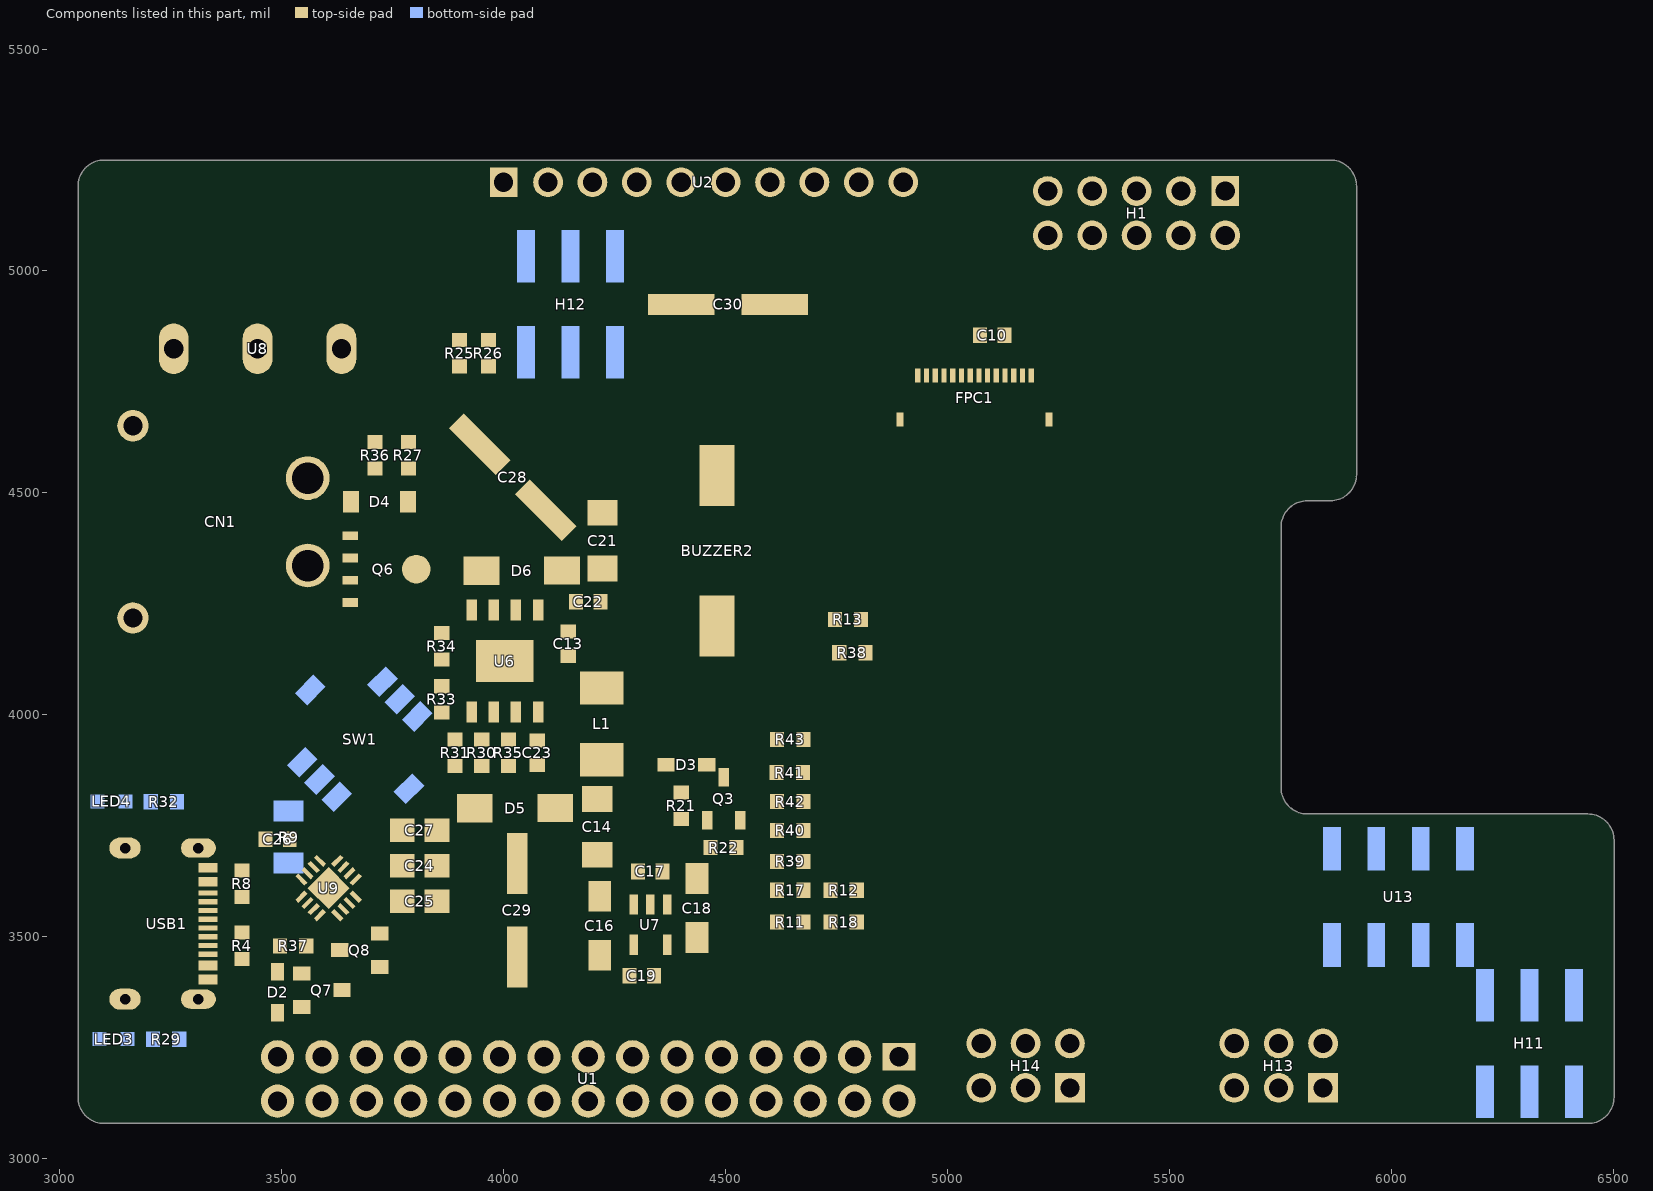
[diagram p0: the components of this part, seen from the top]
# Altium PCB MISC51977.pcbdoc (part 4 of 4)
Units mil, origin at the board's own origin, x right, y up, seen from the top; angles counter-clockwise.
Board outline 3460 x 2170.19 mil, 4 copper layers (Top Layer, VCC, GND, Bottom Layer), stack 62.447 mil thick; 74 components, 60 nets, 282 pads, 462 vias.

## Other copper (continued)
Bottom Layer:
  region net $2N1757: 3177.91,3809.54 3177.91,3799.54 3174.46,3799.22 3171.12,3798.27 3168.01,3796.71 3165.25,3794.61 3162.91,3792.04 3162.91,3817.04 3165.25,3814.47 3168.01,3812.37 3171.12,3810.82 3174.46,3809.86 3177.91,3809.54
  region net $1N29256: 3182.91,3274.92 3182.91,3264.92 3179.46,3264.6 3176.12,3263.64 3173.01,3262.09 3170.25,3259.99 3167.91,3257.42 3167.91,3282.42 3170.25,3279.84 3173.01,3277.74 3176.12,3276.19 3179.46,3275.24 3182.91,3274.92
  region net +5V: 3299.6,3275 3299.6,3265 3296.15,3264.68 3292.81,3263.72 3289.7,3262.17 3286.94,3260.07 3284.6,3257.5 3284.6,3282.5 3286.94,3279.93 3289.7,3277.83 3292.81,3276.28 3296.15,3275.32 3299.6,3275
  region net $1N29256: 3178.53,3264.92 3178.53,3274.92 3181.99,3275.24 3185.33,3276.19 3188.44,3277.74 3191.2,3279.84 3193.53,3282.42 3193.53,3257.42 3191.2,3259.99 3188.44,3262.09 3185.33,3263.64 3181.99,3264.6 3178.53,3264.92
  region net $2N1757: 3173.53,3799.54 3173.53,3809.54 3176.99,3809.86 3180.33,3810.82 3183.44,3812.37 3186.2,3814.47 3188.53,3817.04 3188.53,3792.04 3186.2,3794.61 3183.44,3796.71 3180.33,3798.27 3176.99,3799.22 3173.53,3799.54
  region net 3V3: 3278.97,3826.85 3284.91,3818.65 3282.63,3815.05 3280.97,3811.12 3279.95,3806.99 3279.6,3802.74 3263.06,3821.55 3267.31,3821.89 3271.44,3822.91 3275.37,3824.58 3278.97,3826.85
  region net TX: 4750.32,3262.61 4757.39,3269.68 4759.59,3267.66 4761.66,3266.14 4763.63,3265.04 4765.52,3264.33 4767.36,3263.95 4769.18,3263.86 4771.01,3264 4772.86,3264.32 4776.78,3265.3 4781.14,3266.41 4783.56,3266.87 4786.17,3267.22 4789,3267.39 4792.08,3267.34 4752.66,3227.92 4752.61,3231 4752.78,3233.83 4753.13,3236.44 4753.59,3238.86 4754.7,3243.22 4755.68,3247.14 4756,3248.99 4756.14,3250.82 4756.05,3252.64 4755.67,3254.48 4754.96,3256.37 4753.86,3258.34 4752.34,3260.41
  region net RX: 4732.05,3215.02 4738.75,3194.18 4736.84,3195.89 4734.85,3197.27 4732.8,3198.34 4730.69,3199.13 4728.53,3199.66 4726.31,3199.95 4724.05,3200.03 4721.74,3199.91 4717.01,3199.17 4712.16,3197.93 4707.21,3196.36 4702.19,3194.64 4723.78,3246.05 4724.63,3244.01 4725.27,3241.95 4726.05,3237.82 4726.42,3233.7 4726.67,3229.65 4727.06,3225.71 4727.41,3223.79 4727.9,3221.93 4728.58,3220.11 4729.47,3218.35 4730.61,3216.65
  region net MOTOR_DIR_L: 4550.32,3162.61 4557.39,3169.68 4559.59,3167.66 4561.66,3166.14 4563.63,3165.04 4565.52,3164.33 4567.36,3163.95 4569.18,3163.86 4571.01,3164 4572.86,3164.32 4576.78,3165.3 4581.14,3166.41 4583.56,3166.87 4586.17,3167.22 4589,3167.39 4592.08,3167.34 4552.66,3127.92 4552.61,3131 4552.78,3133.83 4553.13,3136.44 4553.59,3138.86 4554.7,3143.22 4555.68,3147.14 4556,3148.99 4556.14,3150.82 4556.05,3152.64 4555.67,3154.48 4554.96,3156.37 4553.86,3158.34 4552.34,3160.41
  region net MOTOR_DIR_R: 4450.32,3162.61 4457.39,3169.68 4459.59,3167.66 4461.66,3166.14 4463.63,3165.04 4465.52,3164.33 4467.36,3163.95 4469.18,3163.86 4471.01,3164 4472.86,3164.32 4476.78,3165.3 4481.14,3166.41 4483.56,3166.87 4486.17,3167.22 4489,3167.39 4492.08,3167.34 4452.66,3127.92 4452.61,3131 4452.78,3133.83 4453.13,3136.44 4453.59,3138.86 4454.7,3143.22 4455.68,3147.14 4456,3148.99 4456.14,3150.82 4456.05,3152.64 4455.67,3154.48 4454.96,3156.37 4453.86,3158.34 4452.34,3160.41
  region net TFT180_DC: 4350.32,3162.61 4357.39,3169.68 4359.59,3167.66 4361.66,3166.14 4363.63,3165.04 4365.52,3164.33 4367.36,3163.95 4369.18,3163.86 4371.01,3164 4372.86,3164.32 4376.78,3165.3 4381.14,3166.41 4383.56,3166.87 4386.17,3167.22 4389,3167.39 4392.08,3167.34 4352.66,3127.92 4352.61,3131 4352.78,3133.83 4353.13,3136.44 4353.59,3138.86 4354.7,3143.22 4355.68,3147.14 4356,3148.99 4356.14,3150.82 4356.05,3152.64 4355.67,3154.48 4354.96,3156.37 4353.86,3158.34 4352.34,3160.41
  region net TFT180_RES: 4250.32,3262.61 4257.39,3269.68 4259.59,3267.66 4261.66,3266.14 4263.63,3265.04 4265.52,3264.33 4267.36,3263.95 4269.18,3263.86 4271.01,3264 4272.86,3264.32 4276.78,3265.3 4281.14,3266.41 4283.56,3266.87 4286.17,3267.22 4289,3267.39 4292.08,3267.34 4252.66,3227.92 4252.61,3231 4252.78,3233.83 4253.13,3236.44 4253.59,3238.86 4254.7,3243.22 4255.68,3247.14 4256,3248.99 4256.14,3250.82 4256.05,3252.64 4255.67,3254.48 4254.96,3256.37 4253.86,3258.34 4252.34,3260.41
  region net TFT180_SCL: 3850.32,3262.61 3857.39,3269.68 3859.59,3267.66 3861.66,3266.14 3863.63,3265.04 3865.52,3264.33 3867.36,3263.95 3869.18,3263.86 3871.01,3264 3872.86,3264.32 3876.78,3265.3 3881.14,3266.41 3883.56,3266.87 3886.17,3267.22 3889,3267.39 3892.08,3267.34 3852.66,3227.92 3852.61,3231 3852.78,3233.83 3853.13,3236.44 3853.59,3238.86 3854.7,3243.22 3855.68,3247.14 3856,3248.99 3856.14,3250.82 3856.05,3252.64 3855.67,3254.48 3854.96,3256.37 3853.86,3258.34 3852.34,3260.41
  region net TFT180_CS: 3750.32,3262.61 3757.39,3269.68 3759.59,3267.66 3761.66,3266.14 3763.63,3265.04 3765.52,3264.33 3767.36,3263.95 3769.18,3263.86 3771.01,3264 3772.86,3264.32 3776.78,3265.3 3781.14,3266.41 3783.56,3266.87 3786.17,3267.22 3789,3267.39 3792.08,3267.34 3752.66,3227.92 3752.61,3231 3752.78,3233.83 3753.13,3236.44 3753.59,3238.86 3754.7,3243.22 3755.68,3247.14 3756,3248.99 3756.14,3250.82 3756.05,3252.64 3755.67,3254.48 3754.96,3256.37 3753.86,3258.34 3752.34,3260.41
  region net MOTOR_PWM_R: 3622.61,3169.68 3629.68,3162.61 3627.66,3160.41 3626.14,3158.34 3625.04,3156.37 3624.33,3154.48 3623.95,3152.64 3623.86,3150.82 3624,3148.99 3624.32,3147.14 3625.3,3143.22 3626.41,3138.86 3626.87,3136.44 3627.22,3133.83 3627.39,3131 3627.34,3127.92 3587.92,3167.34 3591,3167.39 3593.83,3167.22 3596.44,3166.87 3598.86,3166.41 3603.22,3165.3 3607.14,3164.32 3608.99,3164 3610.82,3163.86 3612.64,3163.95 3614.48,3164.33 3616.37,3165.04 3618.34,3166.14 3620.41,3167.66
  region net TX: 5829.92,3693.27 5829.92,3703.27 5833.38,3703.6 5836.72,3704.55 5839.82,3706.1 5842.59,3708.2 5844.92,3710.77 5844.92,3685.77 5842.59,3688.35 5839.82,3690.45 5836.72,3692 5833.38,3692.95 5829.92,3693.27
  region net RX: 5933.62,3639.15 5937.03,3656.7 5939.61,3659.64 5941.81,3662.87 5943.59,3666.35 5944.92,3670.03 5944.92,3649.06 5939.11,3644.29 5933.62,3639.15
  region net ENCODER_PWM_R: 5139.13,3288.8 5146.2,3295.87 5148.12,3294.11 5149.94,3292.77 5151.67,3291.79 5153.35,3291.15 5154.99,3290.78 5156.61,3290.67 5158.24,3290.75 5159.89,3290.99 5163.39,3291.77 5167.26,3292.66 5171.69,3293.32 5174.17,3293.46 5176.86,3293.41 5141.59,3258.14 5141.54,3260.83 5141.68,3263.31 5142.34,3267.74 5143.23,3271.61 5144.01,3275.11 5144.25,3276.76 5144.33,3278.39 5144.22,3280.01 5143.85,3281.65 5143.21,3283.33 5142.23,3285.06 5140.89,3286.88
  region net $1N14385: 6384.62,3203.31 6385.98,3216.09 6389.59,3213.81 6393.51,3212.15 6397.65,3211.13 6401.89,3210.78 6389.92,3187.4 6389.58,3191.65 6388.56,3195.79 6386.89,3199.71 6384.62,3203.31
  region net $1N4273: 6376.73,3358.27 6376.73,3368.27 6379.88,3368.6 6382.9,3369.56 6385.65,3371.13 6388.03,3373.23 6389.92,3375.77 6389.92,3350.77 6388.03,3353.31 6385.65,3355.41 6382.9,3356.98 6379.88,3357.94 6376.73,3358.27
  region net $1N14409: 6184.62,3203.31 6185.98,3216.09 6189.59,3213.81 6193.51,3212.15 6197.65,3211.13 6201.89,3210.78 6189.92,3187.4 6189.58,3191.65 6188.56,3195.79 6186.89,3199.71 6184.62,3203.31
  region net $1N14395: 6174.92,3358.27 6174.92,3368.27 6178.38,3368.59 6181.72,3369.55 6184.82,3371.1 6187.59,3373.2 6189.92,3375.77 6189.92,3350.77 6187.59,3353.34 6184.82,3355.44 6181.72,3356.99 6178.38,3357.95 6174.92,3358.27
  region net $1N45238: 4014.92,4839.37 4014.92,4849.37 4018.38,4849.69 4021.72,4850.64 4024.82,4852.19 4027.59,4854.29 4029.92,4856.87 4029.92,4831.87 4027.59,4834.44 4024.82,4836.54 4021.72,4838.09 4018.38,4839.04 4014.92,4839.37
  region net $1N45237: 4030.98,4968.91 4024.62,4976.69 4026.89,4980.29 4028.56,4984.21 4029.58,4988.35 4029.92,4992.6 4046.89,4974.22 4042.65,4973.87 4038.51,4972.85 4034.59,4971.19 4030.98,4968.91
  region net KEY_UP: 3724.7,4037.31 3714.7,4037 3713.76,4041.16 3712.16,4045.11 3709.96,4048.76 3707.2,4052 3732.2,4052.31 3729.44,4049.06 3727.23,4045.41 3725.64,4041.46 3724.7,4037.31
  region net KEY_UP: 3760.76,4089.45 3766.84,4079.45 3762.69,4078.51 3758.73,4076.92 3755.09,4074.71 3751.84,4071.95 3745.76,4096.95 3749.01,4094.19 3752.65,4091.99 3756.61,4090.39 3760.76,4089.45
  region net KEY_LEFT: 3845.21,4005 3838.29,3995 3834.14,3994.06 3830.18,3992.47 3826.54,3990.26 3823.29,3987.5 3830.21,4012.5 3833.46,4009.74 3837.11,4007.53 3841.06,4005.94 3845.21,4005
  region net KEY_DOWN: 3664.54,3807.53 3657.47,3800.46 3654.8,3802.68 3651.76,3804.37 3648.47,3805.46 3645.03,3805.94 3641.56,3805.76 3658.3,3822.51 3658.58,3819.2 3659.36,3815.97 3660.64,3812.89 3662.38,3810.06 3664.54,3807.53
  region net KEY_MID: 3618.79,3869.53 3624.87,3859.53 3620.72,3858.59 3616.76,3857 3613.12,3854.79 3609.87,3852.03 3603.79,3877.03 3607.03,3874.27 3610.68,3872.06 3614.63,3870.47 3618.79,3869.53
  region net KEY_RIGHT: 3579.81,3908.5 3585.89,3898.5 3581.73,3897.56 3577.78,3895.96 3574.13,3893.76 3570.89,3891 3564.81,3916 3568.05,3913.24 3571.7,3911.03 3575.65,3909.44 3579.81,3908.5
  region net UD+: 3285,3521.33 3275,3521.33 3274.82,3523.1 3274.31,3525.04 3273.53,3526.87 3272.55,3528.33 3287.45,3528.33 3286.47,3526.87 3285.69,3525.04 3285.18,3523.1
  region net TX: 3605.61,3701.2 3612.68,3694.13 3611.56,3692.75 3610.55,3691.02 3609.81,3689.18 3609.46,3687.45 3598.92,3697.99 3600.65,3698.33 3602.5,3699.08 3604.23,3700.08
  region net $1N5665: 3663.19,3396.41 3678.19,3396.41 3678.1,3394.02 3678.07,3391.88 3678.19,3390.88 3678.46,3389.91 3678.93,3388.95 3679.64,3388.01 3661.74,3388.01 3662.45,3388.95 3662.92,3389.91 3663.19,3390.88 3663.31,3391.88 3663.28,3394.02
  region net $1N5665: 3678.19,3431.99 3663.19,3425.65 3663.28,3427.09 3663.49,3428.44 3663.86,3430.84 3663.84,3431.86 3663.54,3432.75 3662.87,3433.48 3661.74,3434.05 3677.19,3441.92 3676.95,3440.72 3676.94,3439.5 3677.33,3437.01 3677.9,3434.49
  region net KEY_DOWN: 4256.83,3373.49 4246.83,3373.49 4246.65,3375.26 4246.14,3377.19 4245.36,3379.03 4244.38,3380.49 4259.29,3380.49 4258.3,3379.03 4257.53,3377.19 4257.02,3375.26
  region net KEY_DOWN: 4260,3513.67 4270,3513.67 4270.18,3511.9 4270.69,3509.96 4271.47,3508.13 4272.45,3506.67 4257.55,3506.67 4258.53,3508.13 4259.31,3509.96 4259.82,3511.9
  region net MOTOR_PWM_R: 4003.06,3304.36 3995.99,3311.43 3997.11,3312.81 3998.12,3314.54 3998.86,3316.38 3999.2,3318.11 4009.75,3307.57 4008.02,3307.23 4006.17,3306.49 4004.44,3305.48
  region net MOTOR_PWM_R: 4556.33,3595 4556.33,3605 4558.1,3605.18 4560.04,3605.69 4561.87,3606.47 4563.33,3607.45 4563.33,3592.55 4561.87,3593.53 4560.04,3594.31 4558.1,3594.82
  region net KEY_DOWN: 4516.93,3851.8 4509.86,3858.87 4510.98,3860.25 4511.99,3861.98 4512.73,3863.83 4513.08,3865.56 4523.62,3855.02 4521.89,3854.67 4520.04,3853.93 4518.31,3852.92
  region net KEY_UP: 3714.7,4008.44 3724.7,4008.89 3724.89,4007.11 3725.41,4005.17 3726.22,4003.34 3727.25,4001.89 3712.35,4001.44 3713.29,4002.91 3714.03,4004.75 3714.52,4006.68
  region net KEY_RIGHT: 4631.81,3899.09 4638.88,3906.16 4640.26,3905.04 4641.99,3904.03 4643.84,3903.29 4645.57,3902.94 4635.03,3892.4 4634.68,3894.13 4633.94,3895.98 4632.93,3897.71
  region net KEY_MID: 4563.17,3849.76 4570.19,3856.88 4571.57,3855.76 4573.3,3854.75 4575.15,3854.01 4576.89,3853.68 4566.4,3843.09 4566.05,3844.81 4565.3,3846.65 4564.29,3848.38
  region net $1N45238: 4019.73,4849.37 4019.73,4839.37 4017.96,4839.18 4016.02,4838.67 4014.19,4837.89 4012.73,4836.91 4012.73,4851.82 4014.19,4850.84 4016.02,4850.06 4017.96,4849.55
  region net $1N45237: 3956.13,4908.2 3963.2,4901.13 3962.08,4899.75 3961.07,4898.02 3960.33,4896.17 3959.98,4894.44 3949.44,4904.98 3951.17,4905.33 3953.02,4906.07 3954.75,4907.08
  region net I2C_SCL: 5546.33,4760 5546.33,4770 5548.1,4770.18 5550.04,4770.69 5551.87,4771.47 5553.33,4772.45 5553.33,4757.55 5551.87,4758.53 5550.04,4759.31 5548.1,4759.82
  region net $1N14385: 4689.97,3504.64 4689.97,3494.64 4688.2,3494.46 4686.26,3493.95 4684.43,3493.17 4682.97,3492.19 4682.97,3507.09 4684.43,3506.11 4686.26,3505.33 4688.2,3504.82
  region net $1N4273: 6389.86,3368.27 6387.28,3358.27 6385.55,3358.15 6383.66,3357.8 6381.82,3357.24 6380.28,3356.51 6382.86,3371.19 6383.48,3370.53 6384.23,3369.95 6386.02,3369.04 6387.97,3368.47
  region net $1N14395: 6169.65,3368.27 6169.65,3358.27 6167.88,3358.09 6165.95,3357.58 6164.11,3356.8 6162.65,3355.82 6162.65,3370.72 6164.11,3369.74 6165.95,3368.96 6167.88,3368.45
  region net $1N14385: 6268.67,3230 6268.67,3220 6266.9,3219.82 6264.96,3219.31 6263.13,3218.53 6261.67,3217.55 6261.67,3232.45 6263.13,3231.47 6264.96,3230.69 6266.9,3230.18
  region net $1N14385: 4881.61,3494.64 4881.07,3504.64 4882.86,3504.83 4884.8,3505.36 4886.62,3506.17 4888.07,3507.21 4888.61,3492.31 4887.13,3493.24 4885.29,3493.98 4883.36,3494.47
  region net +5V: 3296.33,3265 3296.33,3275 3298.1,3275.18 3300.04,3275.69 3301.87,3276.47 3303.33,3277.45 3303.33,3262.55 3301.87,3263.53 3300.04,3264.31 3298.1,3264.82
  region net KEY_UP: 4736.33,3950 4736.33,3960 4738.1,3960.18 4740.04,3960.69 4741.87,3961.47 4743.33,3962.45 4743.33,3947.55 4741.87,3948.53 4740.04,3949.31 4738.1,3949.82
  region net I2C_SDA: 4695,4003.67 4705,4003.67 4705.18,4001.9 4705.69,3999.96 4706.47,3998.13 4707.45,3996.67 4692.55,3996.67 4693.53,3998.13 4694.31,3999.96 4694.82,4001.9
  region net GND: 4033.67,3400 4033.67,3390 4031.9,3389.82 4029.96,3389.31 4028.13,3388.53 4026.67,3387.55 4026.67,3402.45 4028.13,3401.47 4029.96,3400.69 4031.9,3400.18
  region net 3V3: 3297.71,3831.45 3291.25,3839.13 3292.36,3840.48 3293.39,3842.18 3294.19,3843.98 3294.61,3845.67 3304.52,3834.54 3302.75,3834.28 3300.88,3833.58 3299.12,3832.59
  region net AGND: 3478.67,3535 3478.67,3525 3476.9,3524.82 3474.96,3524.31 3473.13,3523.53 3471.67,3522.55 3471.67,3537.45 3473.13,3536.47 3474.96,3535.69 3476.9,3535.18
  region net GND: 3508.67,3485 3508.67,3475 3506.9,3474.82 3504.96,3474.31 3503.13,3473.53 3501.67,3472.55 3501.67,3487.45 3503.13,3486.47 3504.96,3485.69 3506.9,3485.18
  region net AGND: 3727.15,3621.33 3717.15,3621.33 3716.96,3623.1 3716.45,3625.04 3715.68,3626.87 3714.69,3628.33 3729.6,3628.33 3728.62,3626.87 3727.84,3625.04 3727.33,3623.1
  region net AGND: 3727.15,3584.39 3717.15,3584.39 3716.96,3586.16 3716.45,3588.1 3715.68,3589.93 3714.69,3591.39 3729.6,3591.39 3728.62,3589.93 3727.84,3588.1 3727.33,3586.16
  region net AGND: 3717.15,3611.73 3727.15,3611.73 3727.33,3609.96 3727.84,3608.02 3728.62,3606.19 3729.6,3604.73 3714.69,3604.73 3715.68,3606.19 3716.45,3608.02 3716.96,3609.96
  region net AGND: 3707.32,3555 3707.32,3565 3709.09,3565.18 3711.02,3565.69 3712.85,3566.47 3714.32,3567.45 3714.32,3552.55 3712.85,3553.53 3711.02,3554.31 3709.09,3554.82
  region net AGND: 3717.15,3574.49 3727.15,3572.75 3727.3,3571.03 3727.71,3569.11 3728.35,3567.27 3729.16,3565.75 3714.36,3567.49 3715.51,3568.9 3716.39,3570.7 3716.95,3572.65
  region net GND: 3792.39,3475 3797.68,3485 3801.85,3484.84 3803.72,3484.94 3805.91,3485.42 3799.39,3472.54 3798.92,3473.47 3798.29,3474.14 3797.53,3474.59 3796.65,3474.85 3794.63,3475.02
  region net UD+: 3277.74,3500.19 3288.54,3503.53 3291.1,3501.06 3292.48,3500.01 3294.05,3499.14 3280.46,3493.01 3280.66,3493.97 3280.65,3494.94 3280.46,3495.9 3280.12,3496.85 3279.08,3498.63
  region net TFT180_DC: 5028.87,4686.8 5021.8,4693.87 5022.92,4695.25 5023.93,4696.98 5024.67,4698.83 5025.02,4700.56 5035.56,4690.02 5033.83,4689.67 5031.98,4688.93 5030.25,4687.92
  region net TFT180_CS: 5131.33,4725 5131.33,4735 5133.1,4735.18 5135.04,4735.69 5136.87,4736.47 5138.33,4737.45 5138.33,4722.55 5136.87,4723.53 5135.04,4724.31 5133.1,4724.82
  region net TFFT180_SDA: 5036.33,4805 5036.33,4815 5038.1,4815.18 5040.04,4815.69 5041.87,4816.47 5043.33,4817.45 5043.33,4802.55 5041.87,4803.53 5040.04,4804.31 5038.1,4804.82
  region net I2C_SCL: 4827.71,4200.64 4824.02,4211.09 4825.4,4212.78 4826.51,4214.71 4827.41,4216.77 4828.15,4218.84 4836.98,4203.27 4835.88,4203.41 4834.66,4203.38 4832.06,4202.92 4829.61,4201.97 4828.57,4201.35
  region net I2C_SCL: 4852.49,4224.02 4858.47,4214.02 4857.34,4213.91 4856.13,4213.63 4853.71,4212.58 4851.56,4211.06 4850.71,4210.18 4850.07,4209.24 4844.08,4226.11 4846.09,4225.34 4848.21,4224.67 4850.37,4224.2
  region net I2C_SDA: 4728.07,4155.14 4735.14,4148.07 4734.41,4147.21 4733.79,4146.24 4732.84,4144.02 4732.26,4141.65 4731.99,4139.33 4719.33,4151.99 4721.65,4152.26 4724.02,4152.84 4726.24,4153.79 4727.21,4154.41
  region net KEY_DOWN: 4238.79,3689.14 4243.56,3683.88 4247.79,3678.17 4251.45,3672.07 4254.49,3665.65 4256.88,3658.95 4258.61,3652.06 4259.65,3645.03 4260,3637.93 4270,3635 4270.37,3639.69 4271.47,3644.27 4273.27,3648.62 4275.73,3652.63 4278.79,3656.21 4282.37,3659.27 4286.38,3661.73 4290.73,3663.53 4295.31,3664.63 4300,3665 4297.07,3675 4289.97,3675.35 4282.94,3676.39 4276.05,3678.12 4269.35,3680.51 4262.93,3683.55 4256.83,3687.21 4251.12,3691.44 4245.86,3696.21 4238.79,3689.14
VCC (plane layer: these items are gaps in the copper):
  lines w25: 5015,3055 5015,3350.21 ; 5015,3350.34 5015,3355 4452.22,3355 4442.82,3345.6 4300.51,3345.6 4267.47,3378.65 4267.47,3492.47 4330,3555 4330,3607.23 4566.47,3843.69 4566.47,4231.47 4610,4275 4800,4275 4880,4355 4880,4985 4915,5020 5526.2,5020 5546.48,4999.72 5546.48,3688.52 5787.94,3447.06 5787.94,3050

## Silkscreen, mask and mechanical layers (free items; w line width, h text height)
Top Silkscreen Layer:
  text "scl" at 5640,4590 h80 r90
  text "3v3" at 5345,4585 h80 r90
  text "sda" at 5540,4585 h80 r90
  text "gnd" at 5440,4580 h80 r90
Bottom Silkscreen Layer:
  drawing of 1023 lines, arcs and shapes, not listed
  text "OFF" at 3430,5125 h100
  text "ON" at 3695,5125 h100
  text "o" at 4304.73,5030 h60
  text "SERVO" at 3988.15,4907.76 h40
  text "3v3" at 3290,3835 h80
  text "o" at 6039.73,3700 h60
  text "TX" at 5835,3685 h70
  text "Loongson" at 4325,3420 h220
  text "PWM_L" at 5890,3370 h30
  text "DIR_L" at 6275,3370 h30
  text "o" at 5990,3360 h60
  text "PWM_R" at 5232.88,3318.32 h30
  text "PWM_L" at 5630.7,3317.61 h30
  text "o" at 5065,3310 h60
  text "o" at 5460,3310 h60
  text "o" at 4024.86,3260 h60
  text "MOTOR" at 6345,3235 h40
  text "5V" at 3295,3155 h80
  text "PWM_R" at 5890,3115 h30
  text "DIR_R" at 6280,3115 h30
  text "o" at 4964.73,3095 h60
  text "o" at 3444.73,3085 h60
Mechanical Layer:
  lines w0.1: 4521.42,3395.63 cw(c4555.79,3395.63) 4555.79,3430 5574.41,3430 cw(c5574.41,3395.63) 5608.78,3395.63 cw(c5574.41,3395.63) 5574.41,3361.26 4555.79,3361.26 cw(c4555.79,3395.63) 4521.42,3395.63

## Dimensions
6675,5250 to 6675,3079.81 on Document Layer
6500.6,5455 to 3040.6,5455 on Document Layer
3040.6,4900 to 4770,4900 on Document Layer
5483.31,5249.95 to 5484.98,4204.95 on Document Layer